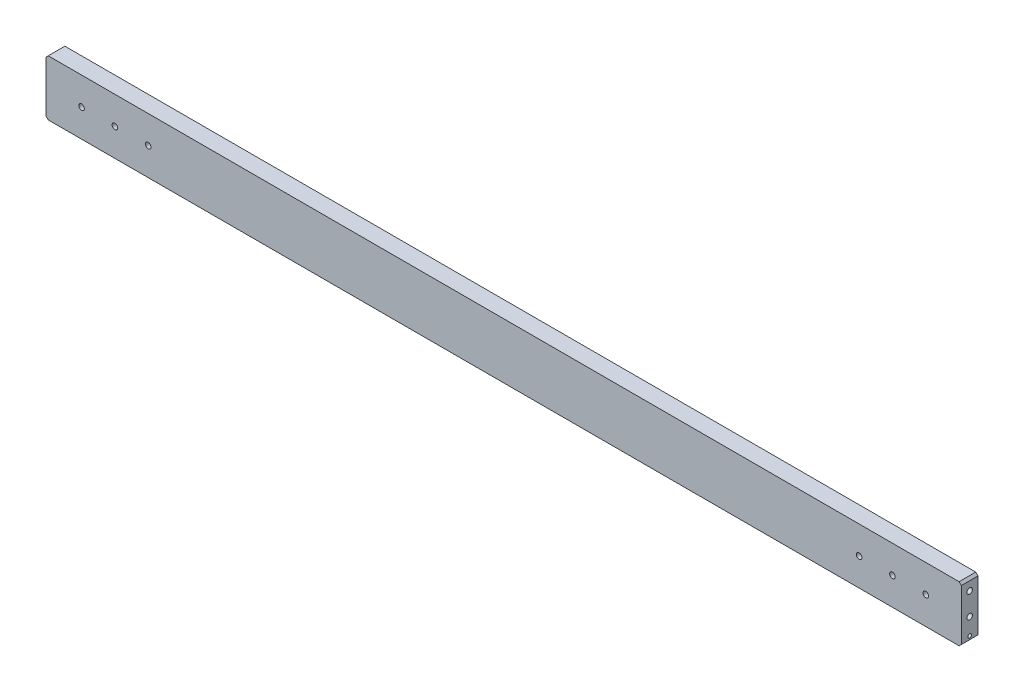
SolidWorks part; units mm, degrees
material "SUS304"
ref_plane "前视基准面" through (0, 0, 0) normal (0, 0, 1) x (1, 0, 0)
ref_plane "上视基准面" through (0, 0, 0) normal (0, 1, 0) x (1, 0, 0)
ref_plane "右视基准面" through (0, 0, 0) normal (1, 0, 0) x (0, 0, -1)
sketch "草图1" plane through (0, 0, 0) normal (0, 0, 1) x (1, 0, 0)
  line L1 (-824, 50) -> (-824, 0)
  line L2 (-824, 50) -> (0, 50)
  line L3 (0, 50) -> (0, 0)
  line L4 (-824, 0) -> (0, 0)
  dimension "D1" = 824
  dimension "D2" = 50
extrude "凸台-拉伸1" add sketch "草图1" along normal blind 15
hole_wizard "M6 螺纹孔1" positions "草图2" profile "草图3" tap size "M6" standard "ISO"
sketch "草图2" plane through (0, 0, 0) normal (1, 0, 0) x (0, -1, 0)
  line L0 (-40, -7.5) -> (-20.0001, -7.5) construction
  line L1 (-20.0001, -7.5) -> (0, -7.5) construction
  line L2 (0, -15) -> (0, 0) construction
  point P0 (-40, -7.5)
  point P2 (-20.0001, -7.5)
  dimension "D1" = 19.9999
  dimension "D2" = 20.0001
sketch "草图3" plane through (0, 40, 7.5) normal (0, 1, 0) x (0, 0, -1)
  line L0 (0, 0) -> (0, 18.5022)
  line L1 (0, 18.5022) -> (2.5, 17)
  line L2 (2.5, 17) -> (2.5, 0)
  line L5 (2.5, 0) -> (0, 0)
  line L10 (0, 18.5022) -> (-2.5, 17) construction
  line L11 (0, -6.35) -> (0, 107.95) construction
  dimension "螺纹孔钻头直径" = 5
  dimension "螺纹孔钻头深度" = 17
  dimension "导头角度" = 118
cosmetic thread "孔螺蚊线1" parameters "D1"=12, "D2"=6
cosmetic thread "孔螺蚊线2" parameters "D1"=12, "D2"=6
hole_wizard "M4 螺纹孔1" positions "草图4" profile "草图5" tap size "M4" standard "ISO"
sketch "草图4" plane through (0, 0, 0) normal (1, 0, 0) x (0, -1, 0)
  line L0 (-5.0002, -7.5) -> (0, -7.5) construction
  line L1 (0, -15) -> (0, 0) construction
  point P0 (-5.0002, -7.5)
  dimension "D1" = 5.0002
sketch "草图5" plane through (0, 5.0002, 7.5) normal (0, 1, 0) x (0, 0, -1)
  line L0 (0, 0) -> (0, 12.4914)
  line L1 (0, 12.4914) -> (1.65, 11.5)
  line L2 (1.65, 11.5) -> (1.65, 0)
  line L5 (1.65, 0) -> (0, 0)
  line L10 (0, 12.4914) -> (-1.65, 11.5) construction
  line L11 (0, -6.35) -> (0, 107.95) construction
  dimension "螺纹孔钻头直径" = 3.3
  dimension "螺纹孔钻头深度" = 11.5
  dimension "导头角度" = 118
cosmetic thread "孔螺蚊线3" parameters "D1"=8, "D2"=4
ref_plane "基准面1" through (-412, 0, 0) normal (1, 0, 0) x (0, -1, 0)
mirror "镜向1" about plane through (-412, 0, 0) normal (1, 0, 0) of "M6 螺纹孔1", "M4 螺纹孔1"
hole_wizard "M6 螺纹孔2" positions "草图8" profile "草图9" tap size "M6" standard "ISO"
sketch "草图8" plane through (0, 0, 0) normal (0, 0, -1) x (-1, 0, 0)
  line L0 (412, 50) -> (412, 116.6817) construction
  line L7 (0, 50) -> (824, 50) construction
  line L9 (0, 25) -> (32, 25) construction
  line L10 (0, 0) -> (0, 50) construction
  line L12 (32, 25) -> (62, 25) construction
  line L13 (62, 25) -> (92, 25) construction
  line L15 (762, 25) -> (732, 25) construction
  line L16 (792, 25) -> (762, 25) construction
  line L17 (824, 25) -> (792, 25) construction
  point P31 (32, 25)
  point P33 (62, 25)
  point P35 (92, 25)
  point P54 (732, 25)
  point P55 (762, 25)
  point P56 (792, 25)
  dimension "D1" = 30
  dimension "D2" = 32
sketch "草图9" plane through (-792, 25, 0) normal (1, 0, 0) x (0, 1, 0)
  line L0 (0, 0) -> (0, 18.5022)
  line L1 (0, 18.5022) -> (2.5, 17)
  line L2 (2.5, 17) -> (2.5, 0)
  line L5 (2.5, 0) -> (0, 0)
  line L10 (0, 18.5022) -> (-2.5, 17) construction
  line L11 (0, -6.35) -> (0, 107.95) construction
  dimension "螺纹孔钻头直径" = 5
  dimension "螺纹孔钻头深度" = 17
  dimension "导头角度" = 118
cosmetic thread "孔螺蚊线20" parameters "D1"=12, "D2"=6
cosmetic thread "孔螺蚊线21" parameters "D1"=12, "D2"=6
cosmetic thread "孔螺蚊线22" parameters "D1"=12, "D2"=6
cosmetic thread "孔螺蚊线23" parameters "D1"=12, "D2"=6
cosmetic thread "孔螺蚊线24" parameters "D1"=12, "D2"=6
cosmetic thread "孔螺蚊线25" parameters "D1"=12, "D2"=6
chamfer "倒角1" distance 2 angle 45 4 edges at (-824, 50, 7.5) (-824, 0, 7.5) (0, 50, 7.5) (0, 0, 7.5)
